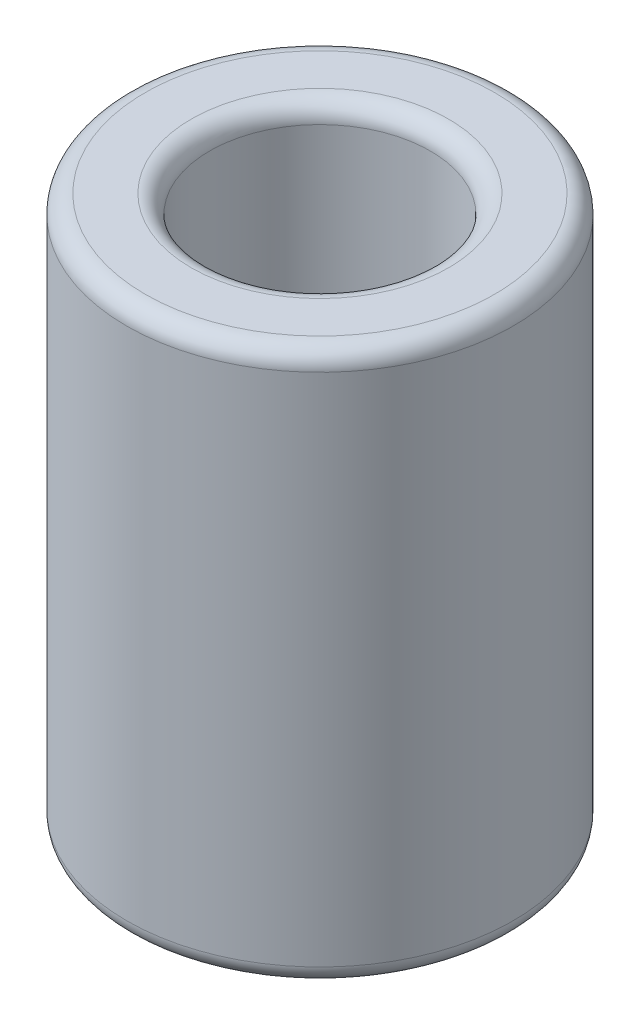
from build123d import *

# Parameters (mm, degrees)
SKETCH1_R           = 10.5
SKETCH1_R_2         = 6
BOSS_EXTRUDE1_DEPTH = 30
FILLET1_R           = 1


with BuildPart() as part:
    # Sketch1 → Boss-Extrude1 (new body)
    with BuildSketch(Plane(origin=(0, 0, 0), x_dir=(1, 0, 0), z_dir=(0, 1, 0))):
        with Locations(Location((0, 0, 0), (0, 0, 270))):
            Circle(SKETCH1_R)
        with Locations(Location((0, 0, 0), (0, 0, 270))):
            Circle(SKETCH1_R_2, mode=Mode.SUBTRACT)
    extrude(amount=BOSS_EXTRUDE1_DEPTH)

    # Fillet1
    fillet1_edges = [part.edges().sort_by_distance(p)[0] for p in [
        (0, 0, -10.5),
        (0, 30, -10.5),
        (0, 0, -6),
        (0, 30, -6),
    ]]
    fillet(fillet1_edges, radius=FILLET1_R)


solid = part.part
